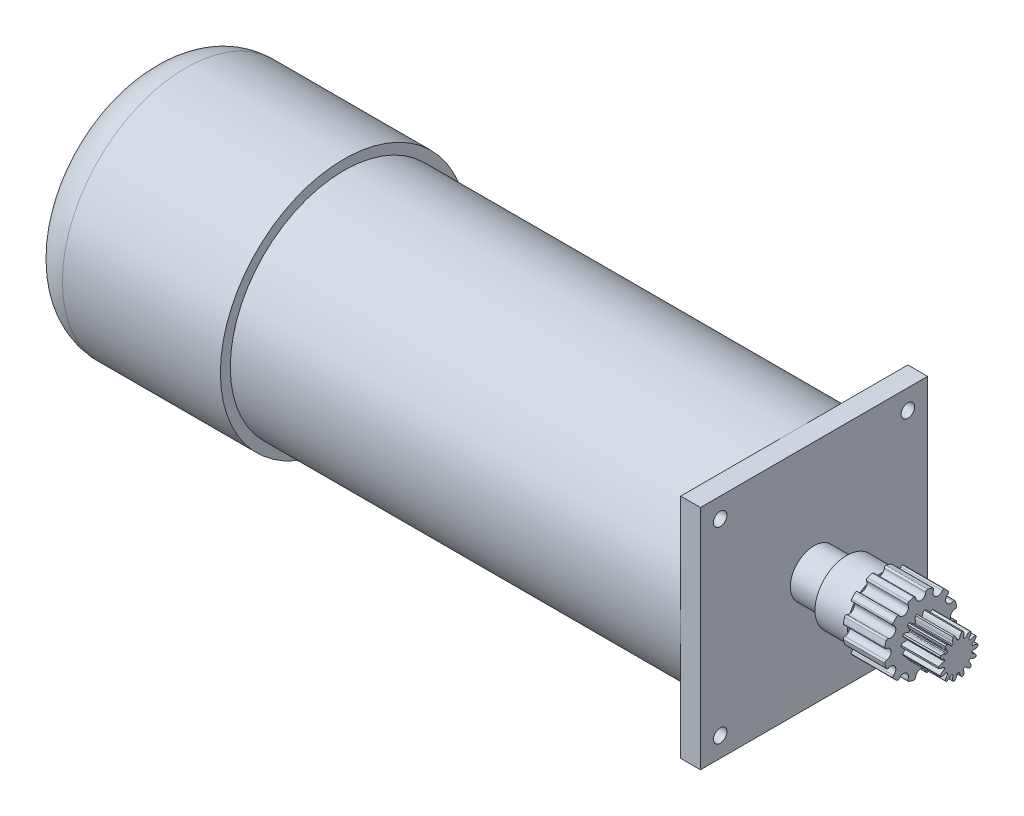
from build123d import *

# Parameters (mm, degrees)
SKETCH_1_R               = 12
EXTRUDE_1_DEPTH          = 16.5
SKETCH_2_R               = 16
EXTRUDE_2_DEPTH          = 16.5
SKETCH_3_R               = 18.5
EXTRUDE_3_DEPTH          = 21
SKETCH_4_R               = 10
EXTRUDE_4_DEPTH          = 19
CUT_EXTRUDE_1_DEPTH      = 19
PATTERN_CIRCULAR_1_COUNT = 14
SKETCH_7_W               = 115
SKETCH_7_H               = 115
EXTRUDE_5_DEPTH          = 10
SKETCH_8_R               = 57.5
EXTRUDE_6_DEPTH          = 228
SKETCH_9_R               = 62.5
EXTRUDE_7_DEPTH          = 100
FILLET_1_R               = 20
HOLE_WIZARD_M8_1_D       = 6.8
HOLE_WIZARD_M8_1_DEPTH   = 19.75
HOLE_WIZARD_M8_1_TIP     = 2.042926105
CUT_EXTRUDE_START        = -21
CUT_EXTRUDE_2_DEPTH      = 21
PATTERN_CIRCULAR_3_COUNT = 12


with BuildPart() as part:
    # 草图1 → 凸台-拉伸1 (new body)
    with BuildSketch(Plane(origin=(0, 0, 0), x_dir=(0, 0, -1), z_dir=(1, 0, 0))):
        Circle(SKETCH_1_R)
    extrude(amount=EXTRUDE_1_DEPTH)

    # 草图2 → 凸台-拉伸2 (add)
    with BuildSketch(Plane(origin=(16.5, 0, 0), x_dir=(0, 0, -1), z_dir=(1, 0, 0))):
        Circle(SKETCH_2_R)
    extrude(amount=EXTRUDE_2_DEPTH)

    # 草图3 → 凸台-拉伸3 (add)
    with BuildSketch(Plane(origin=(33, 0, 0), x_dir=(0, 0, -1), z_dir=(1, 0, 0))):
        with Locations(Location((0, 0, 0), (0, 0, 180))):
            Circle(SKETCH_3_R)
    extrude(amount=EXTRUDE_3_DEPTH)

    # 草图4 → 凸台-拉伸4 (add)
    with BuildSketch(Plane(origin=(54, 0, 0), x_dir=(0, 0, -1), z_dir=(1, 0, 0))):
        Circle(SKETCH_4_R)
    extrude(amount=EXTRUDE_4_DEPTH)

    # 草图5 → 切除-拉伸1 (cut)
    with BuildSketch(Plane(origin=(73, 0, 0), x_dir=(0, 0, -1), z_dir=(1, 0, 0))):
        with BuildLine():
            ThreePointArc((0.255392875, 7.182961139), (0, 7.1875), (-0.255392875, 7.182961139))
            add(Edge.make_bspline(
                [(-0.255392875, 7.182961139), (-0.808325866, 7.435028403), (-0.714686214, 7.896369551), (-0.829586172, 8.314261343), (-0.838461083, 8.344220586), (-0.848931349, 8.377130681), (-0.861115077, 8.412939179), (-0.875132909, 8.451589269), (-0.891102634, 8.493020738), (-0.90914072, 8.537169729), (-0.929361726, 8.583968874), (-0.951878351, 8.63334731), (-0.9768013, 8.685230742), (-1.004239203, 8.739541488), (-1.034298521, 8.796198534), (-1.06708346, 8.855117594), (-1.102695877, 8.91621116), (-1.141235198, 8.979388573), (-1.18279833, 9.044556076), (-1.22747958, 9.111616887), (-1.27537057, 9.18047126), (-1.32656016, 9.251016558), (-1.381134364, 9.32314732), (-1.439176279, 9.39675534), (-1.500766005, 9.471729737), (-1.565980575, 9.547957033), (-1.634893881, 9.625321233), (-1.707576607, 9.703703904), (-1.784096159, 9.78298426), (-1.864516601, 9.863039244), (-1.948898589, 9.943743613), (-2.037299314, 10.024970027), (-2.12977244, 10.106589138), (-2.226368046, 10.188469679), (-2.327132574, 10.270478558), (-2.432108772, 10.35248095), (-2.54133565, 10.434340392), (-2.654848427, 10.515918879), (-2.772678485, 10.59707696), (-2.89485333, 10.67767384), (-3.021396548, 10.757567478), (-3.152327767, 10.836614684), (-3.287662621, 10.914671226), (-3.42741272, 10.991591932), (-3.571585598, 11.067230792), (-3.771679551, 11.167157482), (-3.925467366, 11.238224295), (-4.029884317, 11.284013458)],
                knots=[0, 0, 0, 0, 0.215624359, 0.220482059, 0.225911253, 0.231911941, 0.238484123, 0.245627799, 0.253342969, 0.261629634, 0.270487792, 0.279917445, 0.289918591, 0.300491232, 0.311635367, 0.323350996, 0.335638119, 0.348496736, 0.361926847, 0.375928452, 0.390501552, 0.405646145, 0.421362233, 0.437649814, 0.45450889, 0.47193946, 0.489941524, 0.508515082, 0.527660134, 0.54737668, 0.56766472, 0.588524254, 0.609955283, 0.631957805, 0.654531822, 0.677677333, 0.701394337, 0.725682836, 0.750542829, 0.775974316, 0.801977297, 0.828551773, 0.855697742, 0.883415205, 0.911704163, 0.940564615, 1, 1, 1, 1], degree=3))
            ThreePointArc((-4.029884317, 11.284013458), (0, 11.982025177), (4.029884317, 11.284013458))
            add(Edge.make_bspline(
                [(0.255392875, 7.182961139), (0.808325866, 7.435028403), (0.714686214, 7.896369551), (0.829586172, 8.314261343), (0.838461083, 8.344220586), (0.848931349, 8.377130681), (0.861115077, 8.412939179), (0.875132909, 8.451589269), (0.891102634, 8.493020738), (0.90914072, 8.537169729), (0.929361726, 8.583968874), (0.951878351, 8.63334731), (0.9768013, 8.685230742), (1.004239203, 8.739541488), (1.034298521, 8.796198534), (1.06708346, 8.855117594), (1.102695877, 8.91621116), (1.141235198, 8.979388573), (1.18279833, 9.044556076), (1.22747958, 9.111616887), (1.27537057, 9.18047126), (1.32656016, 9.251016558), (1.381134364, 9.32314732), (1.439176279, 9.39675534), (1.500766005, 9.471729737), (1.565980575, 9.547957033), (1.634893881, 9.625321233), (1.707576607, 9.703703904), (1.784096159, 9.78298426), (1.864516601, 9.863039244), (1.948898589, 9.943743613), (2.037299314, 10.024970027), (2.12977244, 10.106589138), (2.226368046, 10.188469679), (2.327132574, 10.270478558), (2.432108772, 10.35248095), (2.54133565, 10.434340392), (2.654848427, 10.515918879), (2.772678485, 10.59707696), (2.89485333, 10.67767384), (3.021396548, 10.757567478), (3.152327767, 10.836614684), (3.287662621, 10.914671226), (3.42741272, 10.991591932), (3.571585598, 11.067230792), (3.771679551, 11.167157482), (3.925467366, 11.238224295), (4.029884317, 11.284013458)],
                knots=[0, 0, 0, 0, 0.215624359, 0.220482059, 0.225911253, 0.231911941, 0.238484123, 0.245627799, 0.253342969, 0.261629634, 0.270487792, 0.279917445, 0.289918591, 0.300491232, 0.311635367, 0.323350996, 0.335638119, 0.348496736, 0.361926847, 0.375928452, 0.390501552, 0.405646145, 0.421362233, 0.437649814, 0.45450889, 0.47193946, 0.489941524, 0.508515082, 0.527660134, 0.54737668, 0.56766472, 0.588524254, 0.609955283, 0.631957805, 0.654531822, 0.677677333, 0.701394337, 0.725682836, 0.750542829, 0.775974316, 0.801977297, 0.828551773, 0.855697742, 0.883415205, 0.911704163, 0.940564615, 1, 1, 1, 1], degree=3))
        make_face()
    cut_extrude_1 = extrude(amount=-CUT_EXTRUDE_1_DEPTH, mode=Mode.SUBTRACT)

    # 阵列(圆周)1: 切除-拉伸1 ×14 about axis
    pattern_circular_1_axis = Axis((88.99, 0, 0), (-1, 0, 0))
    for i in range(1, PATTERN_CIRCULAR_1_COUNT):
        add(cut_extrude_1.rotate(pattern_circular_1_axis, i * 360 / PATTERN_CIRCULAR_1_COUNT), mode=Mode.SUBTRACT)

    # 草图7 → 凸台-拉伸5 (add)
    with BuildSketch(Plane.ZY):
        Rectangle(SKETCH_7_W, SKETCH_7_H)
    extrude(amount=EXTRUDE_5_DEPTH)

    # 草图8 → 凸台-拉伸6 (add)
    with BuildSketch(Plane.ZY.offset(10)):
        Circle(SKETCH_8_R)
    extrude(amount=EXTRUDE_6_DEPTH)

    # 草图9 → 凸台-拉伸7 (add)
    with BuildSketch(Plane.ZY.offset(238)):
        Circle(SKETCH_9_R)
    extrude(amount=EXTRUDE_7_DEPTH)

    # 圆角1
    fillet_1_edges = [part.edges().sort_by_distance(p)[0] for p in [
        (-338, 0, -62.5),
    ]]
    fillet(fillet_1_edges, radius=FILLET_1_R)

    # M8 螺纹孔1
    with Locations(Plane(origin=(-10, 47.5, -47.5), x_dir=(0, 0, -1), z_dir=(-1, 0, 0))):
        with Locations((0, 0), (-95, 0), (-95, 95), (0, 95)):
            Hole(HOLE_WIZARD_M8_1_D / 2, depth=HOLE_WIZARD_M8_1_DEPTH)
            with Locations((0, 0, -(HOLE_WIZARD_M8_1_DEPTH + HOLE_WIZARD_M8_1_TIP / 2))):  # 118° drill point
                Cone(0, HOLE_WIZARD_M8_1_D / 2, HOLE_WIZARD_M8_1_TIP, mode=Mode.SUBTRACT)

    # 草图11 → 切除-拉伸2 (cut)
    with BuildSketch(Plane(origin=(54, 0, 0), x_dir=(0, 0, -1), z_dir=(1, 0, 0)).offset(CUT_EXTRUDE_START)):
        with BuildLine():
            ThreePointArc((3.518679482, 18.162293212), (0, 18.5), (-3.518679482, 18.162293212))
            ThreePointArc((-3.518679482, 18.162293212), (-2.871619786, 18.005445404), (-2.567346394, 17.413241734))
            ThreePointArc((-2.567346394, 17.413241734), (0, 14.96), (2.567346394, 17.413241734))
            ThreePointArc((2.567346394, 17.413241734), (2.871619786, 18.005445404), (3.518679482, 18.162293212))
        make_face()
    cut_extrude_2 = extrude(amount=CUT_EXTRUDE_2_DEPTH, mode=Mode.SUBTRACT)

    # 阵列(圆周)3: 切除-拉伸2 ×12 about axis
    pattern_circular_3_axis = Axis((0, 0, 0), (1, 0, 0))
    for i in range(1, PATTERN_CIRCULAR_3_COUNT):
        add(cut_extrude_2.rotate(pattern_circular_3_axis, i * 360 / PATTERN_CIRCULAR_3_COUNT), mode=Mode.SUBTRACT)


solid = part.part
